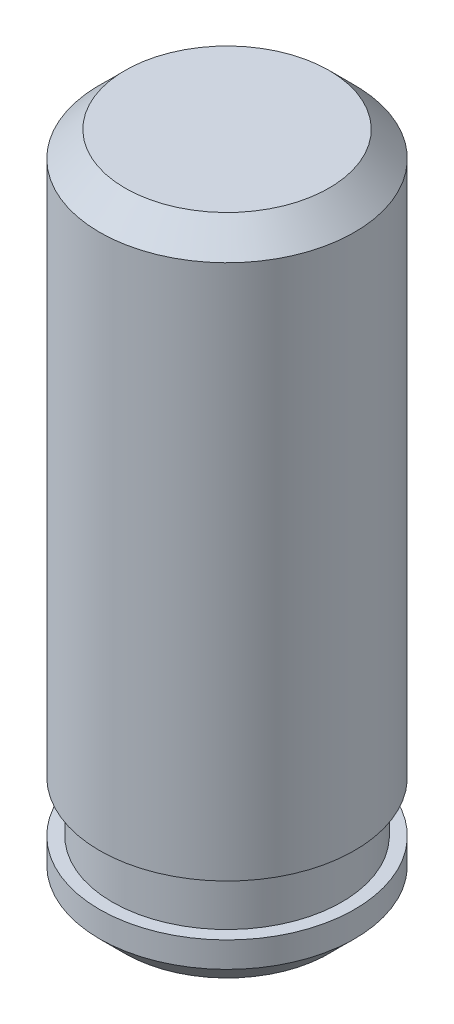
from build123d import *

# Parameters (mm, degrees)
SKETCH1_R           = 2.5
BOSS_EXTRUDE1_DEPTH = 1
SKETCH2_R           = 2.25
BOSS_EXTRUDE2_DEPTH = 1
SKETCH3_R           = 2.5
BOSS_EXTRUDE3_DEPTH = 11
CHAMFER1_SIZE       = 0.5


with BuildPart() as part:
    # Sketch1 → Boss-Extrude1 (new body)
    with BuildSketch(Plane(origin=(0, 0, 0), x_dir=(1, 0, 0), z_dir=(0, 1, 0))):
        with Locations(Location((0, 0, 0), (0, 0, 270))):
            Circle(SKETCH1_R)
    extrude(amount=BOSS_EXTRUDE1_DEPTH)

    # Sketch2 → Boss-Extrude2 (add)
    with BuildSketch(Plane(origin=(0, 1, 0), x_dir=(1, 0, 0), z_dir=(0, 1, 0))):
        with Locations(Location((0, 0, 0), (0, 0, 270))):
            Circle(SKETCH2_R)
    extrude(amount=BOSS_EXTRUDE2_DEPTH)

    # Sketch3 → Boss-Extrude3 (add)
    with BuildSketch(Plane(origin=(0, 2, 0), x_dir=(1, 0, 0), z_dir=(0, 1, 0))):
        with Locations(Location((0, 0, 0), (0, 0, 270))):
            Circle(SKETCH3_R)
    extrude(amount=BOSS_EXTRUDE3_DEPTH)

    # Chamfer1
    chamfer1_edges = [part.edges().sort_by_distance(p)[0] for p in [
        (0, 13, -2.5),
        (0, 0, -2.5),
    ]]
    chamfer(chamfer1_edges, length=CHAMFER1_SIZE)


solid = part.part
